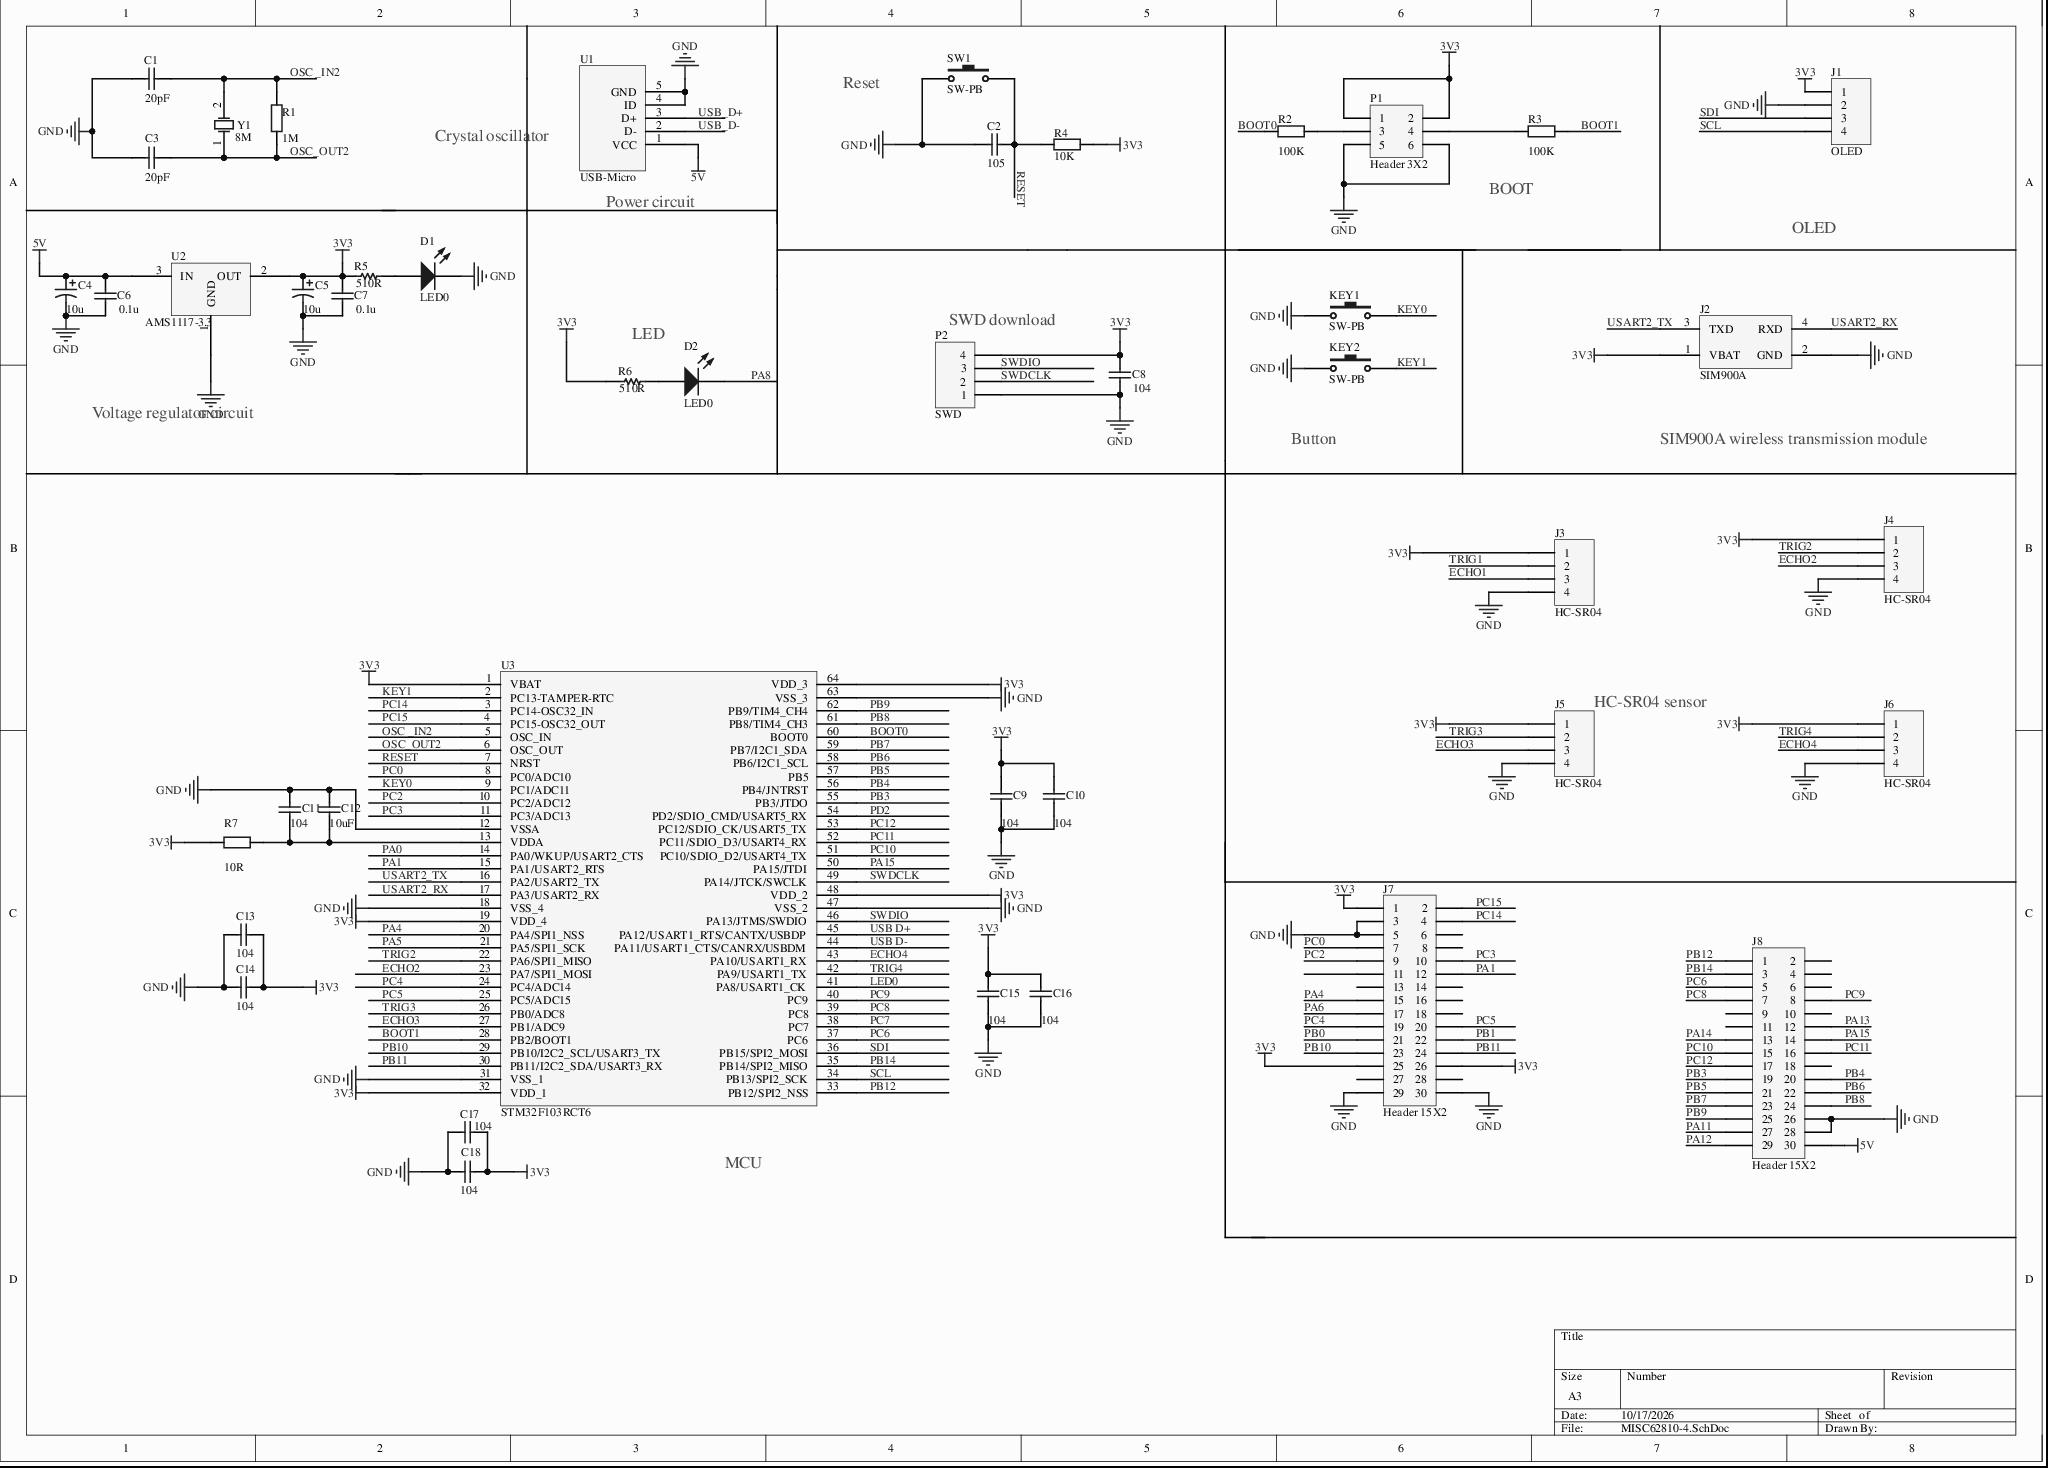
[diagram p0: MISC62810-4.SchDoc]
# Altium project MISC62810-4.PrjPcb
1 sheet, 44 parts. Net scope: global (net labels, ports and power ports of the same name join across sheets).
Board file: MISC62810.PcbDoc

## Sheet MISC62810-4.SchDoc
size A3

### Parts
C1  value 20pF  [C 0805_L]  (hidden comment: Cap)
C2  value 105  [C 0805_L]
C3  value 20pF  [C 0805_L]  (hidden comment: Cap)
C4  value 10u  [CM A(3*5.4)]  (hidden comment: Cap Pol1)
C5  value 10u  [CM A(3*5.4)]  (hidden comment: Cap Pol1)
C6  value 0.1u  [C 0805_L]  (hidden comment: Cap)
C7  value 0.1u  [C 0805_L]  (hidden comment: Cap)
C8  value 104  [C 0805_L]  (hidden comment: Cap)
C9  value 104  [C 0805_L]  (hidden comment: Cap)
C10  value 104  [C 0805_L]  (hidden comment: Cap)
C11  value 104  [C 0805_L]  (hidden comment: Cap)
C12  value 10uF  [C 0805_L]  (hidden comment: Cap)
C13  value 104  [C 0805_L]  (hidden comment: Cap)
C14  value 104  [C 0805_L]  (hidden comment: Cap)
C15  value 104  [C 0805_L]  (hidden comment: Cap)
C16  value 104  [C 0805_L]  (hidden comment: Cap)
C17  value 104  [C 0805_L]  (hidden comment: Cap)
C18  value 104  [C 0805_L]  (hidden comment: Cap)
D1  LED0  [LED 0805G]
D2  LED0  [LED 0805G]
J1  OLED  [0.96OLED_4P]
J2  SIM900A  [HDR1X4]
J3  HC-SR04  [HDR1X4]
J4  HC-SR04  [HDR1X4]
J5  HC-SR04  [HDR1X4]
J6  HC-SR04  [HDR1X4]
J7  Header 15X2  [HDR2X15]
J8  Header 15X2  [HDR2X15]
KEY1  SW-PB  [TSW SMD-3*4*2.5]
KEY2  SW-PB  [TSW SMD-3*4*2.5]
P1  Header 3X2  [HDR2X3]
P2  SWD  [HDR1X4]
R1  value 1M  [R 0805_L]
R2  value 100K  [R 0805_L]  (hidden comment: Res2)
R3  value 100K  [R 0805_L]  (hidden comment: Res2)
R4  value 10K  [R 0805_L]  (hidden comment: Res2)
R5  value 510R  [R 0805_L]  (hidden comment: Res1)
R6  value 510R  [R 0805_L]  (hidden comment: Res1)
R7  value 10R  [R 0805_L]  (hidden comment: Res2)
SW1  SW-PB  [TSW SMD-3*4*2.5]
U1  USB-Micro  [USB-MICRO_B]
U2  AMS1117-3.3  [SOT223]
U3  STM32F103RCT6  [LQFP64 7x7]
Y1  8M  [OSC 5032-2P]

### Nets
3V3: C5.1 C7.2 C8.2 C9.2 C10.2 C13.1 C14.1 C15.2 C16.2 C17.2 C18.2 J1.1 J2.1(VBAT) J3.1 J4.1 J5.1 J6.1 J7.1 J7.25 J7.26 P1.1 P1.2 P2.4 R4.2 R5.1 R6.1 R7.1 U2.2(OUT) U3.1(VBAT) U3.19(VDD_4) U3.32(VDD_1) U3.48(VDD_2) U3.64(VDD_3)
5V: C4.1 C6.2 J8.30 U1.1(VCC) U2.3(IN)
GND: C1.1 C2.1 C3.1 C4.2 C5.2 C6.1 C7.1 C8.1 C9.1 C10.1 C11.2 C12.2 C13.2 C14.2 C15.1 C16.1 C17.1 C18.1 D1.2(K) J1.2 J2.2(GND) J3.4 J4.4 J5.4 J6.4 J7.3 J7.5 J7.29 J7.30 J8.26 J8.28 KEY1.1 KEY2.1 P1.5 P1.6 P2.1 SW1.1 U1.4(ID) U1.5(GND) U2.1(GND) U3.12(VSSA) U3.18(VSS_4) U3.31(VSS_1) U3.47(VSS_2) U3.63(VSS_3)
BOOT0: R2.1 U3.60(BOOT0)
BOOT1: R3.2 U3.28(PB2/BOOT1)
ECHO1: J3.3
ECHO2: J4.3 U3.23(PA7/SPI1_MOSI)
ECHO3: J5.3 U3.27(PB1/ADC9)
ECHO4: J6.3 U3.43(PA10/USART1_RX)
KEY0: KEY1.2 U3.9(PC1/ADC11)
KEY1: KEY2.2 U3.2(PC13-TAMPER-RTC)
LED0: U3.41(PA8/USART1_CK)
OSC _IN2: C1.2 R1.2 U3.5(OSC_IN) Y1.2(OSC2)
OSC_OUT2: C3.2 R1.1 U3.6(OSC_OUT) Y1.1(OSC1)
PA0: U3.14(PA0/WKUP/USART2_CTS)
PA1: J7.12 U3.15(PA1/USART2_RTS)
PA4: J7.15 U3.20(PA4/SPI1_NSS)
PA5: U3.21(PA5/SPI1_SCK)
PA6: J7.17
PA8: D2.2(K)
PA11: J8.27
PA12: J8.29
PA13: J8.12
PA14: J8.13
PA15: J8.14 U3.50(PA15/JTDI)
PB0: J7.21
PB1: J7.22
PB3: J8.19 U3.55(PB3/JTDO)
PB4: J8.20 U3.56(PB4/JNTRST)
PB5: J8.21 U3.57(PB5)
PB6: J8.22 U3.58(PB6/I2C1_SCL)
PB7: J8.23 U3.59(PB7/I2C1_SDA)
PB8: J8.24 U3.61(PB8/TIM4_CH3)
PB9: J8.25 U3.62(PB9/TIM4_CH4)
PB10: J7.23 U3.29(PB10/I2C2_SCL/USART3_TX)
PB11: J7.24 U3.30(PB11/I2C2_SDA/USART3_RX)
PB12: J8.1 U3.33(PB12/SPI2_NSS)
PB14: J8.3 U3.35(PB14/SPI2_MISO)
PC0: J7.7 U3.8(PC0/ADC10)
PC2: J7.9 U3.10(PC2/ADC12)
PC3: J7.10 U3.11(PC3/ADC13)
PC4: J7.19 U3.24(PC4/ADC14)
PC5: J7.20 U3.25(PC5/ADC15)
PC6: J8.5 U3.37(PC6)
PC7: U3.38(PC7)
PC8: J8.7 U3.39(PC8)
PC9: J8.8 U3.40(PC9)
PC10: J8.15 U3.51(PC10/SDIO_D2/USART4_TX)
PC11: J8.16 U3.52(PC11/SDIO_D3/USART4_RX)
PC12: J8.17 U3.53(PC12/SDIO_CK/USART5_TX)
PC14: J7.4 U3.3(PC14-OSC32_IN)
PC15: J7.2 U3.4(PC15-OSC32_OUT)
PD2: U3.54(PD2/SDIO_CMD/USART5_RX)
RESET: C2.2 R4.1 SW1.2 U3.7(NRST)
SCL: J1.4 U3.34(PB13/SPI2_SCK)
SDI: J1.3 U3.36(PB15/SPI2_MOSI)
SWDCLK: P2.2 U3.49(PA14/JTCK/SWCLK)
SWDIO: P2.3 U3.46(PA13/JTMS/SWDIO)
TRIG1: J3.2
TRIG2: J4.2 U3.22(PA6/SPI1_MISO)
TRIG3: J5.2 U3.26(PB0/ADC8)
TRIG4: J6.2 U3.42(PA9/USART1_TX)
USART2_RX: J2.4(RXD) U3.17(PA3/USART2_RX)
USART2_TX: J2.3(TXD) U3.16(PA2/USART2_TX)
USB D+: U3.45(PA12/USART1_RTS/CANTX/USBDP)
USB D-: U3.44(PA11/USART1_CTS/CANRX/USBDM)
USB_D+: U1.3(D+)
USB_D-: U1.2(D-)
NetC11_1: C11.1 C12.1 R7.2 U3.13(VDDA)
NetD1_1: D1.1(A) R5.2
NetD2_1: D2.1(A) R6.2
NetP1_3: P1.3 R2.2
NetP1_4: P1.4 R3.1

Not connected (* = marked no-connect by the designer): J7 6* 8* 11* 13* 14* 16* 18* 27* 28*; J8 2* 4* 6* 9* 10* 11* 18*

### Notes on the sheet
- Reset
- Crystal oscillator
- (near U1) Power circuit
- BOOT
- OLED
- LED
- (near P2) SWD download
- Voltage regulator circuit
- Button
- SIM900A wireless transmission module
- (near J5) HC-SR04 sensor
- MCU

### Library data of the parts
C1-C3 C6-C18 = Cap: Capacitor; Published: 8-Jun-2000; LatestRevisionDate: 17-Jul-2002; LatestRevisionNote: Re-released for DXP Platform.; PackageReference: RAD-0.3; PackageDescription: Radial Cap, Thru-Hole; 2 Leads; 0.3 in Pin Spacing; Publisher: Altium Limited
C4 C5 = Cap Pol1: Polarized Capacitor (Radial); Published: 8-Jun-2000; LatestRevisionDate: 17-Jul-2002; LatestRevisionNote: Re-released for DXP Platform.; PackageReference: RB7.6-15; PackageDescription: Polarized Capacitor (Radial); 2 Leads; Publisher: Altium Limited
D1 D2 = LED0: Typical INFRARED GaAs LED; Published: 8-Jun-2000; LatestRevisionDate: 08-Jul-2005; LatestRevisionNote: Mech Layer 1 removed.; PackageReference: LED-0; PackageDescription: LED; 2 Leads; Publisher: Altium Limited
J1 J3-J6 P2 = Header 4: Header, 4-Pin; LatestRevisionDate: 17-Jul-2002; LatestRevisionNote: Re-released for DXP Platform.; Publisher: Altium Limited
J2 U1-U3 = Component_1
J7 J8 = Header 15X2: Header, 15-Pin, Dual row; LatestRevisionDate: 17-Jul-2002; LatestRevisionNote: Re-released for DXP Platform.; Publisher: Altium Limited
KEY1 KEY2 SW1 = SW-PB: Switch; Published: 24-Mar-1999; LatestRevisionDate: 17-Jul-2002; LatestRevisionNote: Re-released for DXP Platform.; PackageReference: SPST-2; PackageDescription: Switch; 2 Leads; Publisher: Altium Limited
P1 = Header 3X2: Header, 3-Pin, Dual row; LatestRevisionDate: 17-Jul-2002; LatestRevisionNote: Re-released for DXP Platform.; Publisher: Altium Limited
R1-R4 R7 = Res2: Resistor; Published: 8-Jun-2000; LatestRevisionDate: 17-Jul-2002; LatestRevisionNote: Re-released for DXP Platform.; PackageReference: AXIAL-0.4; PackageDescription: Axial Device, Thru-Hole; 2 Leads; 0.4 in Pin Spacing; Publisher: Altium Limited
R5 R6 = Res1: Resistor; Published: 8-Jun-2000; LatestRevisionDate: 17-Jul-2002; LatestRevisionNote: Re-released for DXP Platform.; PackageReference: AXIAL-0.3; PackageDescription: Axial Device, Thru-Hole; 2 Leads; 0.3 in Pin Spacing; Publisher: Altium Limited
Y1 = XTAL: Crystal Oscillator; Published: 8-Jun-2000; LatestRevisionDate: 17-Jul-2002; LatestRevisionNote: Re-released for DXP Platform.; PackageReference: R38; PackageDescription: Crystal, Thru-Hole; 2 Leads; Body 3.1 x 8.2 mm (Dia.xH); Publisher: Altium Limited